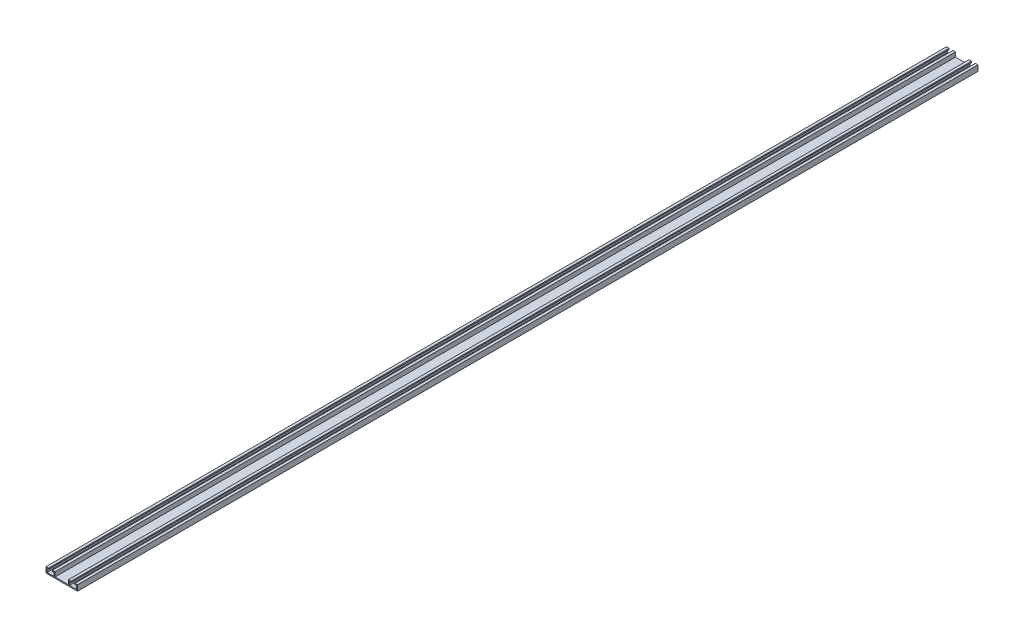
from build123d import *

# Parameters (mm, degrees)
EXTRUDE_1_DEPTH        = 800
SKETCH_2_W             = 6
SKETCH_2_H             = 1
EXTRUDE_2_DEPTH        = 800
HOLE_WIZARD_M3_1_D     = 3.4
HOLE_WIZARD_M3_1_DEPTH = 1


with BuildPart() as part:
    # 草图1 → 拉伸-薄壁1 (new body)
    with BuildSketch(Plane.XY):
        Polygon((2.35, 5), (0, 5), (0, 0), (8, 0), (8, 5), (5.65, 5), (5.65, 4), (7, 4), (7, 1), (1, 1), (1, 4), (2.35, 4), align=None)
    extrude(amount=EXTRUDE_1_DEPTH)

    # 草图2 → 拉伸-薄壁2 (add)
    with BuildSketch(Plane.XY.offset(800)):
        with Locations((-3, 0.5)):
            Rectangle(SKETCH_2_W, SKETCH_2_H)
    extrude(amount=-EXTRUDE_2_DEPTH)

    # 镜向1: part across plane


with BuildPart() as part_1:
    add(part.part)
    add(part.part.mirror(Plane(origin=(-6, 0, -6.08276253), x_dir=(0, 0, 1), z_dir=(1, 0, 0))))

    # M3 间隙孔1
    with Locations(Plane(origin=(0, 1, 0), x_dir=(1, 0, 0), z_dir=(0, 1, 0))):
        with Locations((-16, -10), (-16, -790)):
            Hole(HOLE_WIZARD_M3_1_D / 2, depth=HOLE_WIZARD_M3_1_DEPTH)


solid = part_1.part
